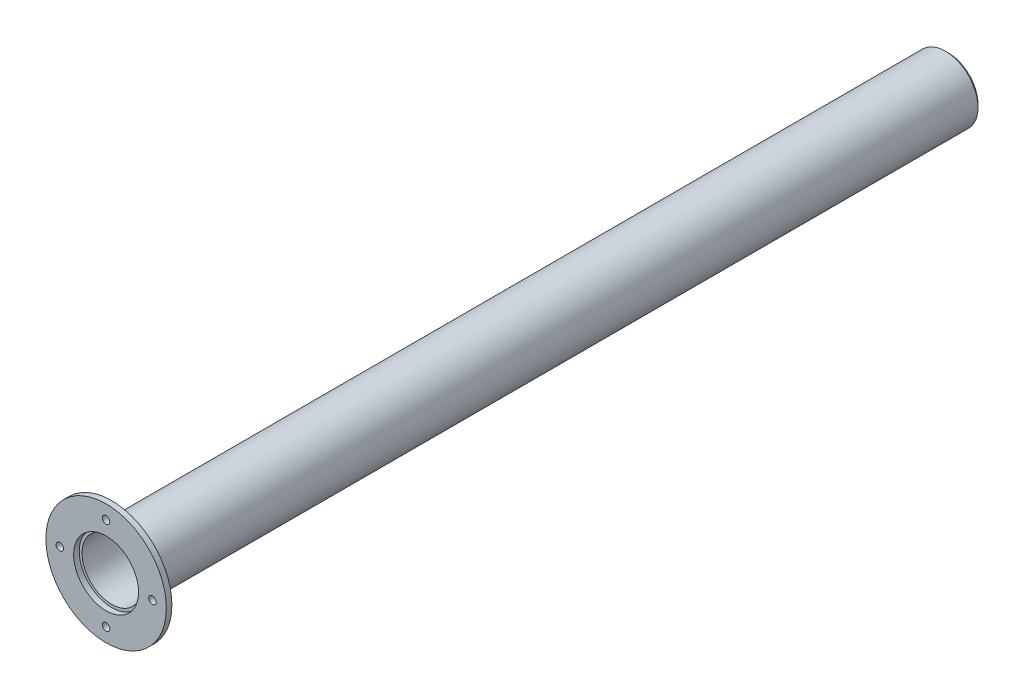
SolidWorks part; units mm, degrees
material "Q235B"
ref_plane "Front" through (0, 0, 0) normal (0, 0, 1) x (1, 0, 0)
ref_plane "Top" through (0, 0, 0) normal (0, 1, 0) x (1, 0, 0)
ref_plane "Right" through (0, 0, 0) normal (1, 0, 0) x (0, 0, -1)
sketch "Sketch1" plane through (0, 0, 0) normal (0, 0, 1) x (1, 0, 0)
  circle A0 centre (0, 0) radius 35
  dimension "D1" = 70
extrude "Thin Extrude1" add sketch "Sketch1" along normal blind 900 thin thin type one direction reverse wall 3
sketch "Sketch3" plane through (0, 0, 0) normal (0, 0, -1) x (-1, 0, 0)
  circle A0 centre (0, 0) radius 32
extrude "Boss-Extrude1" add sketch "Sketch3" along normal blind 3 separate body
sketch "Sketch4" plane through (0, 0, 900) normal (0, 0, 1) x (1, 0, 0)
  circle A0 centre (0, 0) radius 65
  circle A1 centre (0, 0) radius 35
  circle A2 centre (0, 0) radius 35
  dimension "D1" = 0
  dimension "D2" = 30
extrude "Boss-Extrude2" add sketch "Sketch4" along normal blind 6 separate body
sketch "Sketch5" plane through (0, 0, 906) normal (0, 0, 1) x (1, 0, 0)
  circle A0 centre (0, 0) radius 50 construction
  point P3 (0, 50)
  point P4 (-50, 0)
  point P5 (0, -50)
  point P6 (50, 0)
  dimension "D1" = 100
hole_wizard "Ø8.0 (8) Hole1" positions "Sketch7" profile "Sketch6" hole size "Ø8.0" standard "GB" end condition up to next
sketch "Sketch7" plane through (0, 0, 906) normal (0, 0, 1) x (1, 0, 0)
  point P0 (0, 50)
  point P3 (-50, 0)
  point P6 (0, -50)
  point P9 (50, 0)
sketch "Sketch6" plane through (0, 50, 906) normal (1, 0, 0) x (0, -1, 0)
  line L0 (0, 0) -> (0, 6.001)
  line L1 (0, 6.001) -> (4, 6.001)
  line L2 (4, 6.001) -> (4, 0)
  line L5 (4, 0) -> (0, 0)
  line L11 (0, -6.35) -> (0, 107.95) construction
  dimension "通孔孔直径" = 8
  dimension "通孔孔深度" = 6.001
equation "\"零件重量\"= IIF ( \"SW-质量\" > 100 , int ( \"SW-质量\" ) , \"SW-质量\" )"
